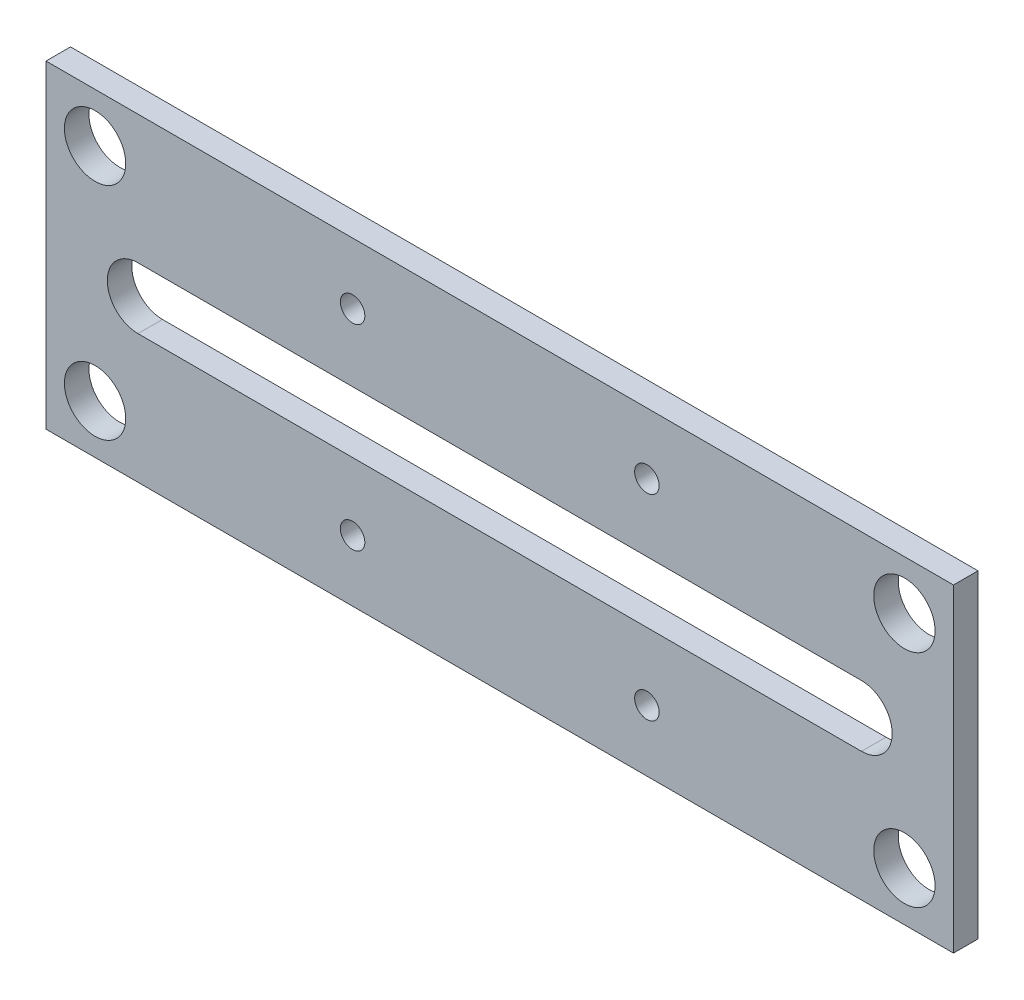
from build123d import *

# Parameters (mm, degrees)
SKETCH1_W            = 370
SKETCH1_H            = 130
SKETCH1_R            = 12.5
BOSS_EXTRUDE1_DEPTH  = 10
M8_CLEARANCE_HOLE1_D = 10


with BuildPart() as part:
    # Sketch1 → Boss-Extrude1 (new body)
    with BuildSketch(Plane(origin=(0, 0, 0), x_dir=(-1, 0, 0), z_dir=(0, 0, -1))):
        with Locations((-185, 65)):
            Rectangle(SKETCH1_W, SKETCH1_H)
        with Locations(Location((-350, 20, 0), (0, 0, 180))):
            Circle(SKETCH1_R, mode=Mode.SUBTRACT)
        with Locations(Location((-20, 110, 0), (0, 0, 180))):
            Circle(SKETCH1_R, mode=Mode.SUBTRACT)
        with Locations(Location((-350, 110, 0), (0, 0, 180))):
            Circle(SKETCH1_R, mode=Mode.SUBTRACT)
        with Locations(Location((-20, 20, 0), (0, 0, 180))):
            Circle(SKETCH1_R, mode=Mode.SUBTRACT)
        with BuildLine():
            Line((-37.5, 52.5), (-332.5, 52.5))
            ThreePointArc((-332.5, 52.5), (-345, 65), (-332.5, 77.5))
            Line((-332.5, 77.5), (-37.5, 77.5))
            ThreePointArc((-37.5, 77.5), (-25, 65), (-37.5, 52.5))
        make_face(mode=Mode.SUBTRACT)
    extrude(amount=-BOSS_EXTRUDE1_DEPTH)

    # M8 Clearance Hole1 (through all)
    with Locations(Plane(origin=(0, 0, 0), x_dir=(-1, 0, 0), z_dir=(0, 0, -1))):
        with Locations((-245, 25), (-125, 25), (-125, 105), (-245, 105)):
            Hole(M8_CLEARANCE_HOLE1_D / 2)


solid = part.part
